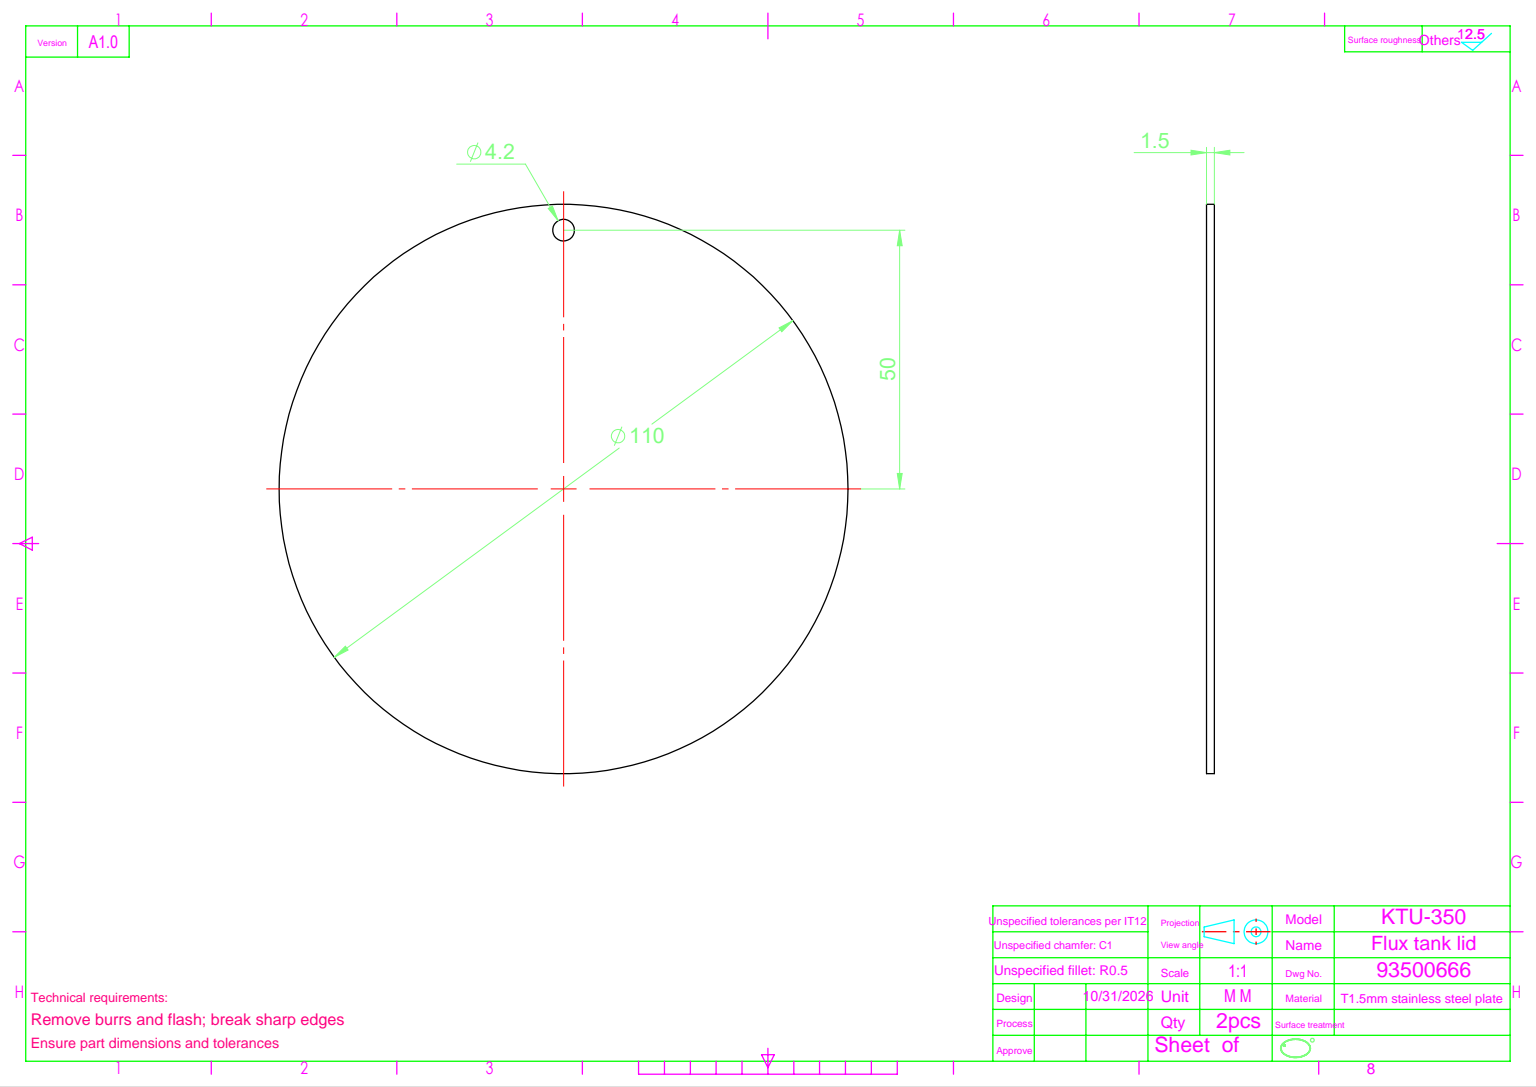
from build123d import *

# Parameters (mm, degrees)
SKETCH_1_R          = 55
EXTRUDE_1_DEPTH     = 1.5
SKETCH_2_R          = 2.1
CUT_EXTRUDE_1_DEPTH = 1.5


with BuildPart() as part:
    # 草图1 → 凸台-拉伸1 (new body)
    with BuildSketch(Plane.XY):
        Circle(SKETCH_1_R)
    extrude(amount=EXTRUDE_1_DEPTH)

    # 草图2 → 切除-拉伸1 (cut)
    with BuildSketch(Plane.XY.offset(1.5)):
        with Locations((0, 50)):
            Circle(SKETCH_2_R)
    extrude(amount=-CUT_EXTRUDE_1_DEPTH, mode=Mode.SUBTRACT)


solid = part.part
